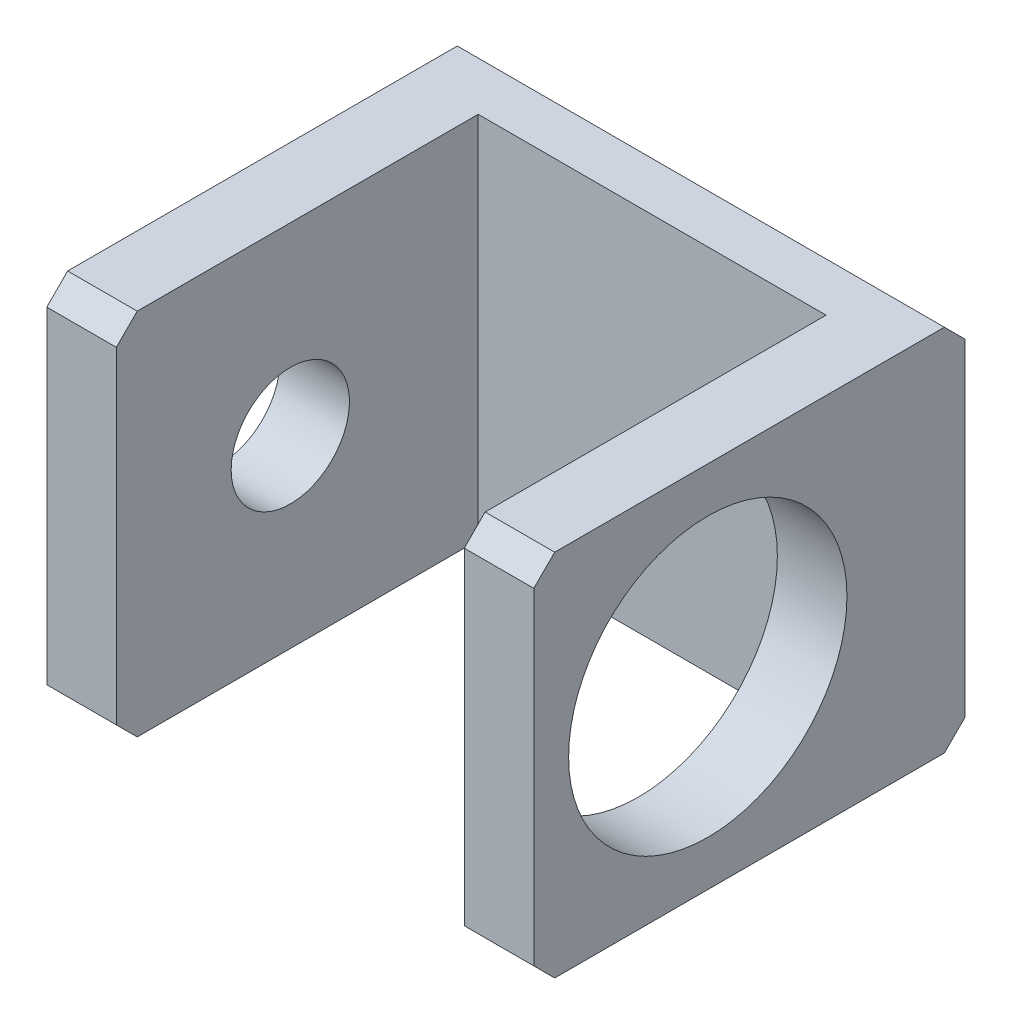
SolidWorks part; units mm, degrees
ref_plane "前视基准面" through (0, 0, 0) normal (0, 0, 1) x (1, 0, 0)
ref_plane "上视基准面" through (0, 0, 0) normal (0, 1, 0) x (1, 0, 0)
ref_plane "右视基准面" through (0, 0, 0) normal (1, 0, 0) x (0, 0, -1)
sketch "草图1" plane through (0, 0, 0) normal (0, 1, 0) x (1, 0, 0)
  line L0 (0, 0) -> (0, 52)
  line L1 (0, 52) -> (50, 52)
  line L2 (50, 52) -> (50, 0)
  line L3 (0, 0) -> (-10, 0)
  line L4 (-10, 0) -> (-10, 62)
  line L5 (-10, 62) -> (60, 62)
  line L6 (60, 62) -> (60, 0)
  line L7 (60, 0) -> (50, 0)
  dimension "D1" = 52
  dimension "D2" = 50
  dimension "D3" = 10
  dimension "D4" = 10
  dimension "D5" = 10
extrude "凸台-拉伸1" add sketch "草图1" along normal mid plane 53
sketch "草图7" plane through (-10, 0, 0) normal (-1, 0, 0) x (0, 0, 1)
  circle A0 centre (-25, 0) radius 8.5
  dimension "D1" = 17
  dimension "D2" = 25
extrude "切除-拉伸2" cut sketch "草图7" against normal up to next
sketch "草图8" plane through (50, 0, 0) normal (-1, 0, 0) x (0, 0, 1)
  circle A0 centre (-25, 0) radius 20
  dimension "D1" = 40
extrude "切除-拉伸3" cut sketch "草图8" against normal up to next
sketch "草图9" plane through (60, 0, 0) normal (1, 0, 0) x (0, 0, -1)
  line L0 (0, 1) -> (5.025, 1)
  line L1 (0, 26.5) -> (0, -26.5) construction
  line L2 (5.025, 1) -> (5.025, -1)
  line L3 (5.025, -1) -> (0, -1)
  line L4 (0, -1) -> (0, 1)
  circle A0 centre (25, 0) radius 20 construction
  dimension "D1" = 2
extrude "切除-拉伸4" [suppressed] cut sketch "草图9" against normal up to next
chamfer "倒角1" [suppressed] distance 1 angle 45
sketch "草图10" [suppressed] plane through (0, 26.5, 0) normal (0, 1, 0) x (1, 0, 0)
  line L1 (60, 1) -> (60, 60) construction
  line L2 (60, 0) -> (50, 0) construction
  circle A0 centre (55, 5) radius 3
  dimension "D1" = 6
  dimension "D2" = 5
  dimension "D3" = 5
extrude "切除-拉伸5" [suppressed] cut sketch "草图10" against normal up to next
hole_wizard "M5 螺纹孔1" positions "3D草图1" profile "草图11" tap size "M5" standard "GB"
sketch3d "3D草图1" [suppressed]
  circle A0 centre (55, 26.5, -5) radius 3 construction
  point P0 (55, -1, -5)
  point P4 (55, 29.5, -5)
sketch "草图11" plane through (55, -1, -5) normal (1, 0, 0) x (0, 0, 1)
  line L0 (0, 0) -> (0, 25.5)
  line L1 (0, 25.5) -> (2.1, 25.5)
  line L2 (2.1, 25.5) -> (2.1, 0)
  line L5 (2.1, 0) -> (0, 0)
  line L11 (0, -6.35) -> (0, 107.95) construction
  dimension "通孔螺纹孔钻头直径" = 4.2
  dimension "通孔螺纹孔钻头深度" = 25.5
cosmetic thread "孔螺蚊线1" parameters "D2"=5
chamfer "倒角2" distance 3 angle 45 2 edges at (25, 26.5, -62) (25, -26.5, -62)
chamfer "倒角3" distance 3 angle 45 4 edges at (55, 26.5, 0) (55, -26.5, 0) (-5, -26.5, 0) (-5, 26.5, 0)
